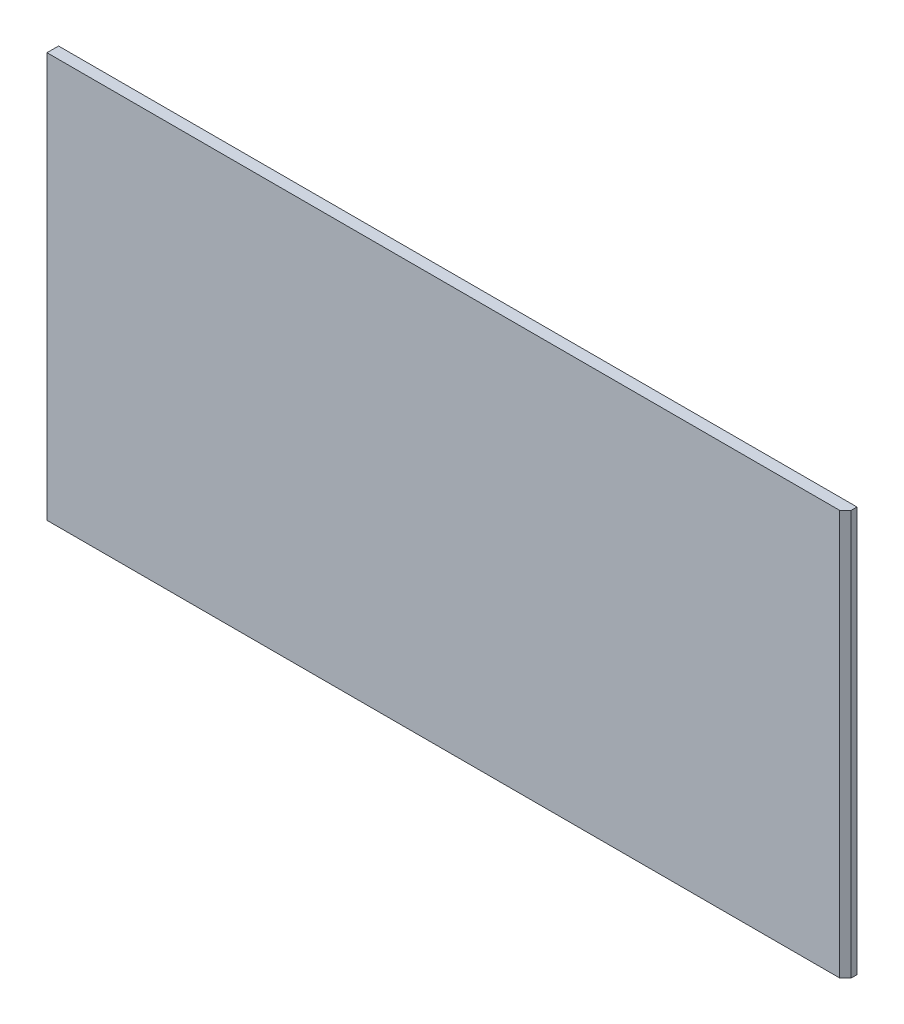
SolidWorks part; units mm, degrees
material "Q235"
ref_plane "Front Plane" through (0, 0, 0) normal (0, 0, 1) x (1, 0, 0)
ref_plane "Top Plane" through (0, 0, 0) normal (0, 1, 0) x (1, 0, 0)
ref_plane "Right Plane" through (0, 0, 0) normal (1, 0, 0) x (0, 0, -1)
sketch "Sketch1" plane through (0, 0, 0) normal (0, 0, 1) x (1, 0, 0)
  line L1 (0, 0) -> (1380, 0)
  line L2 (0, 0) -> (0, 700)
  line L3 (0, 700) -> (1380, 700)
  line L4 (1380, 0) -> (1380, 700)
  dimension "D1" = 1380
  dimension "D2" = 700
extrude "Boss-Extrude1" add sketch "Sketch1" along normal blind 20
chamfer "Chamfer1" distance 10 angle 45 1 edges at (1380, 350, 20)
